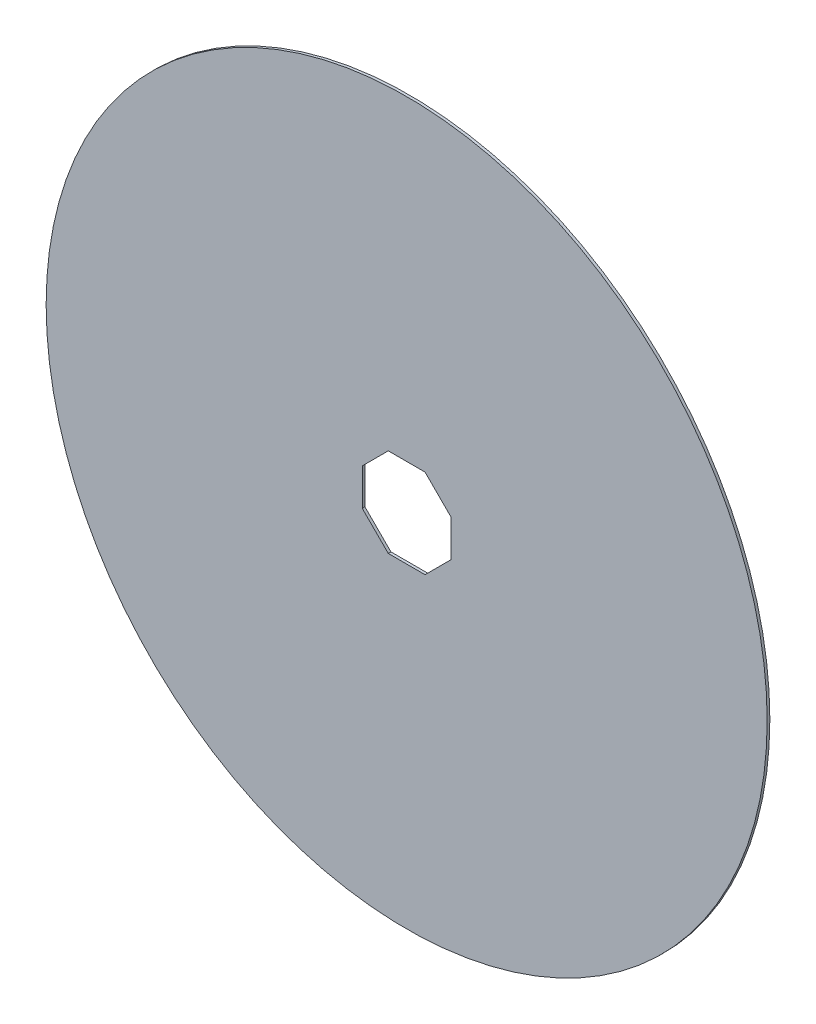
SolidWorks part; units mm, degrees
ref_plane "前视基准面" through (0, 0, 0) normal (0, 0, 1) x (1, 0, 0)
ref_plane "上视基准面" through (0, 0, 0) normal (0, 1, 0) x (1, 0, 0)
ref_plane "右视基准面" through (0, 0, 0) normal (1, 0, 0) x (0, 0, -1)
sketch "草图1" plane through (0, 0, 0) normal (0, 0, 1) x (1, 0, 0)
  line L0 (33.2597, 13.7766) -> (13.7766, 33.2597)
  line L13 (-13.7766, 33.2597) -> (-33.2597, 13.7766)
  line L14 (-33.2597, 13.7766) -> (-33.2597, -13.7766)
  line L15 (-33.2597, -13.7766) -> (-13.7766, -33.2597)
  line L16 (-13.7766, -33.2597) -> (13.7766, -33.2597)
  line L17 (13.7766, -33.2597) -> (33.2597, -13.7766)
  line L18 (33.2597, -13.7766) -> (33.2597, 13.7766)
  line L19 (13.7766, 33.2597) -> (-13.7766, 33.2597)
  circle A0 centre (0, 0) radius 270
  circle A2 centre (0, 0) radius 33.2597 construction
  dimension "D1" = 72
extrude "凸台-拉伸1" add sketch "草图1" along normal blind 2
